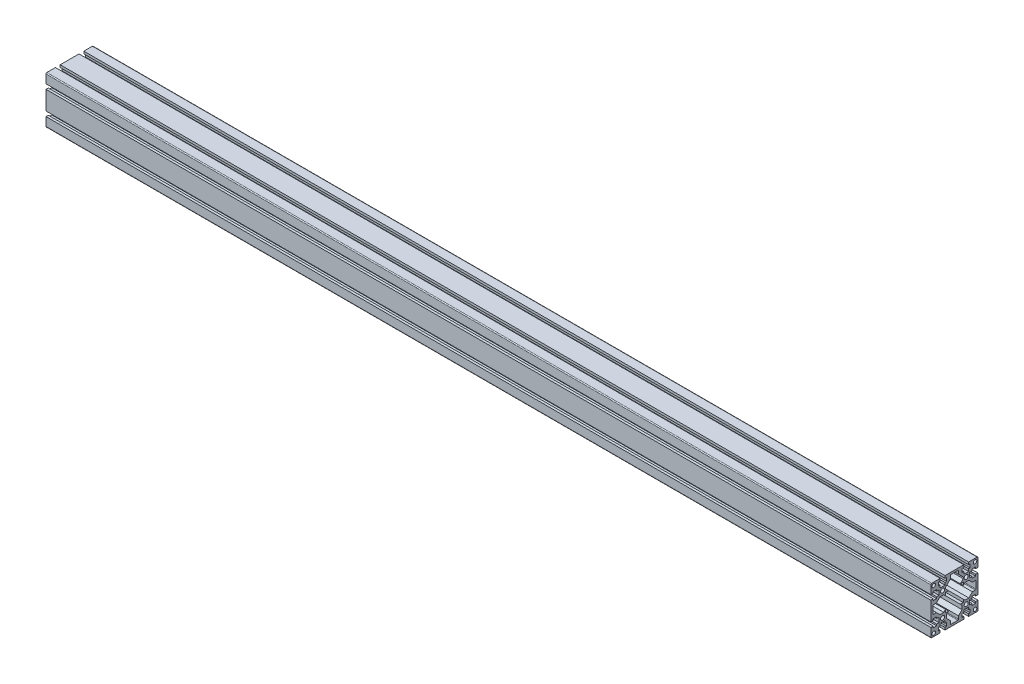
from build123d import *

# Parameters (mm, degrees)
SKETCH1_R                                 = 3.4
SKETCH1_R_2                               = 3
ALUMINIUM_PROFILE_80_X_80G_X_R1_5_1_DEPTH = 1500
SKETCH10_R                                = 3
CUT_EXTRUDE1_DEPTH                        = 1502.066287677


with BuildPart() as part:
    # Sketch1 → Aluminium profile 80 X 80G X R1.5(1) (new body)
    with BuildSketch(Plane.YZ.offset(-530.344827586)):
        with BuildLine():
            Line((-24.05, 40), (-24.05, 36))
            Line((-24.05, 36), (-26.75, 36))
            Line((-26.75, 36), (-26.75, 30))
            Line((-26.75, 30), (-24.05, 30))
            Line((-24.05, 30), (-24.05, 26))
            Line((-24.05, 26), (-15.95, 26))
            Line((-15.95, 26), (-15.95, 30))
            Line((-15.95, 30), (-13.25, 30))
            Line((-13.25, 30), (-13.25, 36))
            Line((-13.25, 36), (-15.95, 36))
            Line((-15.95, 36), (-15.95, 40))
            Line((-15.95, 40), (15.95, 40))
            Line((15.95, 40), (15.95, 36))
            Line((15.95, 36), (13.25, 36))
            Line((13.25, 36), (13.25, 30))
            Line((13.25, 30), (15.95, 30))
            Line((15.95, 30), (15.95, 26))
            Line((15.95, 26), (24.05, 26))
            Line((24.05, 26), (24.05, 30))
            Line((24.05, 30), (26.75, 30))
            Line((26.75, 30), (26.75, 36))
            Line((26.75, 36), (24.05, 36))
            Line((24.05, 36), (24.05, 40))
            Line((24.05, 40), (38.5, 40))
            ThreePointArc((38.5, 40), (39.560660172, 39.560660172), (40, 38.5))
            Line((40, 38.5), (40, 24.05))
            Line((40, 24.05), (36, 24.05))
            Line((36, 24.05), (36, 26.75))
            Line((36, 26.75), (30, 26.75))
            Line((30, 26.75), (30, 24.05))
            Line((30, 24.05), (26, 24.05))
            Line((26, 24.05), (26, 15.95))
            Line((26, 15.95), (30, 15.95))
            Line((30, 15.95), (30, 13.25))
            Line((30, 13.25), (36, 13.25))
            Line((36, 13.25), (36, 15.95))
            Line((36, 15.95), (40, 15.95))
            Line((40, 15.95), (40, -15.95))
            Line((40, -15.95), (36, -15.95))
            Line((36, -15.95), (36, -13.25))
            Line((36, -13.25), (30, -13.25))
            Line((30, -13.25), (30, -15.95))
            Line((30, -15.95), (26, -15.95))
            Line((26, -15.95), (26, -24.05))
            Line((26, -24.05), (30, -24.05))
            Line((30, -24.05), (30, -26.75))
            Line((30, -26.75), (36, -26.75))
            Line((36, -26.75), (36, -24.05))
            Line((36, -24.05), (40, -24.05))
            Line((40, -24.05), (40, -38.5))
            ThreePointArc((40, -38.5), (39.560660172, -39.560660172), (38.5, -40))
            Line((38.5, -40), (24.05, -40))
            Line((24.05, -40), (24.05, -36))
            Line((24.05, -36), (26.75, -36))
            Line((26.75, -36), (26.75, -30))
            Line((26.75, -30), (24.05, -30))
            Line((24.05, -30), (24.05, -26))
            Line((24.05, -26), (15.95, -26))
            Line((15.95, -26), (15.95, -30))
            Line((15.95, -30), (13.25, -30))
            Line((13.25, -30), (13.25, -36))
            Line((13.25, -36), (15.95, -36))
            Line((15.95, -36), (15.95, -40))
            Line((15.95, -40), (-15.95, -40))
            Line((-15.95, -40), (-15.95, -36))
            Line((-15.95, -36), (-13.25, -36))
            Line((-13.25, -36), (-13.25, -30))
            Line((-13.25, -30), (-15.95, -30))
            Line((-15.95, -30), (-15.95, -26))
            Line((-15.95, -26), (-24.05, -26))
            Line((-24.05, -26), (-24.05, -30))
            Line((-24.05, -30), (-26.75, -30))
            Line((-26.75, -30), (-26.75, -36))
            Line((-26.75, -36), (-24.05, -36))
            Line((-24.05, -36), (-24.05, -40))
            Line((-24.05, -40), (-38.5, -40))
            ThreePointArc((-38.5, -40), (-39.560660172, -39.560660172), (-40, -38.5))
            Line((-40, -38.5), (-40, -24.05))
            Line((-40, -24.05), (-36, -24.05))
            Line((-36, -24.05), (-36, -26.75))
            Line((-36, -26.75), (-30, -26.75))
            Line((-30, -26.75), (-30, -24.05))
            Line((-30, -24.05), (-26, -24.05))
            Line((-26, -24.05), (-26, -15.95))
            Line((-26, -15.95), (-30, -15.95))
            Line((-30, -15.95), (-30, -13.25))
            Line((-30, -13.25), (-36, -13.25))
            Line((-36, -13.25), (-36, -15.95))
            Line((-36, -15.95), (-40, -15.95))
            Line((-40, -15.95), (-40, 15.95))
            Line((-40, 15.95), (-36, 15.95))
            Line((-36, 15.95), (-36, 13.25))
            Line((-36, 13.25), (-30, 13.25))
            Line((-30, 13.25), (-30, 15.95))
            Line((-30, 15.95), (-26, 15.95))
            Line((-26, 15.95), (-26, 24.05))
            Line((-26, 24.05), (-30, 24.05))
            Line((-30, 24.05), (-30, 26.75))
            Line((-30, 26.75), (-36, 26.75))
            Line((-36, 26.75), (-36, 24.05))
            Line((-36, 24.05), (-40, 24.05))
            Line((-40, 24.05), (-40, 38.5))
            ThreePointArc((-40, 38.5), (-39.560660172, 39.560660172), (-38.5, 40))
            Line((-38.5, 40), (-24.05, 40))
        make_face()
        with Locations((-20, 20)):
            Circle(SKETCH1_R, mode=Mode.SUBTRACT)
        with Locations((20, 20)):
            Circle(SKETCH1_R, mode=Mode.SUBTRACT)
        with Locations((20, -20)):
            Circle(SKETCH1_R, mode=Mode.SUBTRACT)
        with Locations((-20, -20)):
            Circle(SKETCH1_R, mode=Mode.SUBTRACT)
        with Locations((-35, 35)):
            Circle(SKETCH1_R_2, mode=Mode.SUBTRACT)
        with Locations((35, 35)):
            Circle(SKETCH1_R_2, mode=Mode.SUBTRACT)
        with Locations((35, -35)):
            Circle(SKETCH1_R_2, mode=Mode.SUBTRACT)
        with BuildLine():
            Line((-13, 18), (-10, 15))
            Line((-10, 15), (-15, 15))
            Line((-15, 15), (-15, 10))
            Line((-15, 10), (-18, 13))
            Line((-18, 13), (-24.5, 13))
            Line((-24.5, 13), (-30.5, 7))
            Line((-30.5, 7), (-35.5, 7))
            ThreePointArc((-35.5, 7), (-36.207106781, 6.707106781), (-36.5, 6))
            Line((-36.5, 6), (-36.5, -6))
            ThreePointArc((-36.5, -6), (-36.207106781, -6.707106781), (-35.5, -7))
            Line((-35.5, -7), (-30.5, -7))
            Line((-30.5, -7), (-24.5, -13))
            Line((-24.5, -13), (-18, -13))
            Line((-18, -13), (-15, -10))
            Line((-15, -10), (-15, -15))
            Line((-15, -15), (-10, -15))
            Line((-10, -15), (-13, -18))
            Line((-13, -18), (-13, -24.5))
            Line((-13, -24.5), (-7, -30.5))
            Line((-7, -30.5), (-7, -35.5))
            ThreePointArc((-7, -35.5), (-6.707106781, -36.207106781), (-6, -36.5))
            Line((-6, -36.5), (6, -36.5))
            ThreePointArc((6, -36.5), (6.707106781, -36.207106781), (7, -35.5))
            Line((7, -35.5), (7, -30.5))
            Line((7, -30.5), (13, -24.5))
            Line((13, -24.5), (13, -18))
            Line((13, -18), (10, -15))
            Line((10, -15), (15, -15))
            Line((15, -15), (15, -10))
            Line((15, -10), (20, -15))
            Line((20, -15), (22.5, -15))
            Line((22.5, -15), (30.5, -7))
            Line((30.5, -7), (35.5, -7))
            ThreePointArc((35.5, -7), (36.207106781, -6.707106781), (36.5, -6))
            Line((36.5, -6), (36.5, 6))
            ThreePointArc((36.5, 6), (36.207106781, 6.707106781), (35.5, 7))
            Line((35.5, 7), (30.5, 7))
            Line((30.5, 7), (22.5, 15))
            Line((22.5, 15), (20, 15))
            Line((20, 15), (15, 10))
            Line((15, 10), (15, 15))
            Line((15, 15), (10, 15))
            Line((10, 15), (13, 18))
            Line((13, 18), (13, 24.5))
            Line((13, 24.5), (7, 30.5))
            Line((7, 30.5), (7, 35.5))
            ThreePointArc((7, 35.5), (6.707106781, 36.207106781), (6, 36.5))
            Line((6, 36.5), (-6, 36.5))
            ThreePointArc((-6, 36.5), (-6.707106781, 36.207106781), (-7, 35.5))
            Line((-7, 35.5), (-7, 30.5))
            Line((-7, 30.5), (-13, 24.5))
            Line((-13, 24.5), (-13, 18))
        make_face(mode=Mode.SUBTRACT)
    extrude(amount=ALUMINIUM_PROFILE_80_X_80G_X_R1_5_1_DEPTH)

    # Sketch10 → Cut-Extrude1 (cut, through all)
    with BuildSketch(Plane(origin=(969.655172414, 0, 0), x_dir=(0, 0, -1), z_dir=(1, 0, 0))):
        with Locations((35, -35)):
            Circle(SKETCH10_R)
    extrude(amount=-CUT_EXTRUDE1_DEPTH, mode=Mode.SUBTRACT)


solid = part.part
